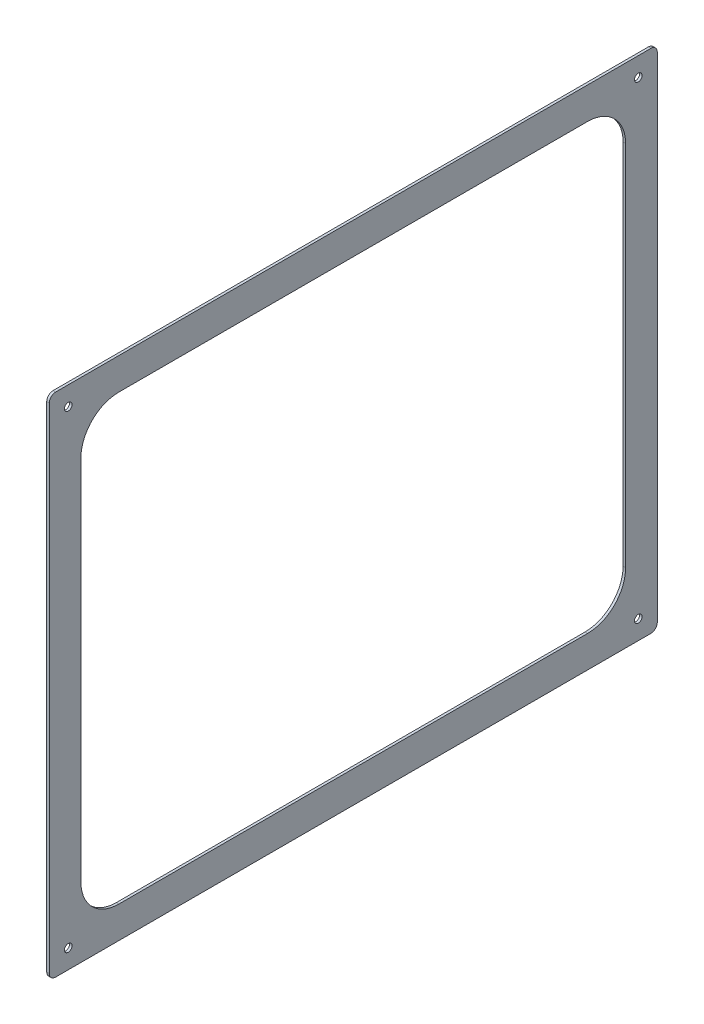
from build123d import *

# Parameters (mm, degrees)
SKETCH_1_W          = 480
SKETCH_1_H          = 400
EXTRUDE_1_DEPTH     = 2
SKETCH_2_R          = 3
CUT_EXTRUDE_1_DEPTH = 313.416388815
FILLET_1_R          = 5
SKETCH_3_W          = 430
SKETCH_3_H          = 350
CUT_EXTRUDE_2_DEPTH = 313.416388815
FILLET_2_R          = 30


with BuildPart() as part:
    # 草图1 → 凸台-拉伸1 (new body)
    with BuildSketch(Plane(origin=(0, 0, 0), x_dir=(0, 0, -1), z_dir=(1, 0, 0))):
        Rectangle(SKETCH_1_W, SKETCH_1_H)
    extrude(amount=EXTRUDE_1_DEPTH)

    # 草图2 → 切除-拉伸1 (cut, through all)
    with BuildSketch(Plane(origin=(2, 0, 0), x_dir=(0, 0, -1), z_dir=(1, 0, 0))):
        with Locations((-225, 185)):
            Circle(SKETCH_2_R)
        with Locations((225, 185)):
            Circle(SKETCH_2_R)
        with Locations((-225, -185)):
            Circle(SKETCH_2_R)
        with Locations((225, -185)):
            Circle(SKETCH_2_R)
    extrude(amount=-CUT_EXTRUDE_1_DEPTH, mode=Mode.SUBTRACT)

    # 圆角1
    fillet_1_edges = [part.edges().sort_by_distance(p)[0] for p in [
        (1, 200, 240),
        (1, 200, -240),
        (1, -200, -240),
        (1, -200, 240),
    ]]
    fillet(fillet_1_edges, radius=FILLET_1_R)

    # 草图3 → 切除-拉伸2 (cut, through all)
    with BuildSketch(Plane(origin=(2, 0, 0), x_dir=(0, 0, -1), z_dir=(1, 0, 0))):
        Rectangle(SKETCH_3_W, SKETCH_3_H)
    extrude(amount=-CUT_EXTRUDE_2_DEPTH, mode=Mode.SUBTRACT)

    # 圆角2
    fillet_2_edges = [part.edges().sort_by_distance(p)[0] for p in [
        (1, -175, 215),
        (1, 175, 215),
        (1, 175, -215),
        (1, -175, -215),
    ]]
    fillet(fillet_2_edges, radius=FILLET_2_R)


solid = part.part
